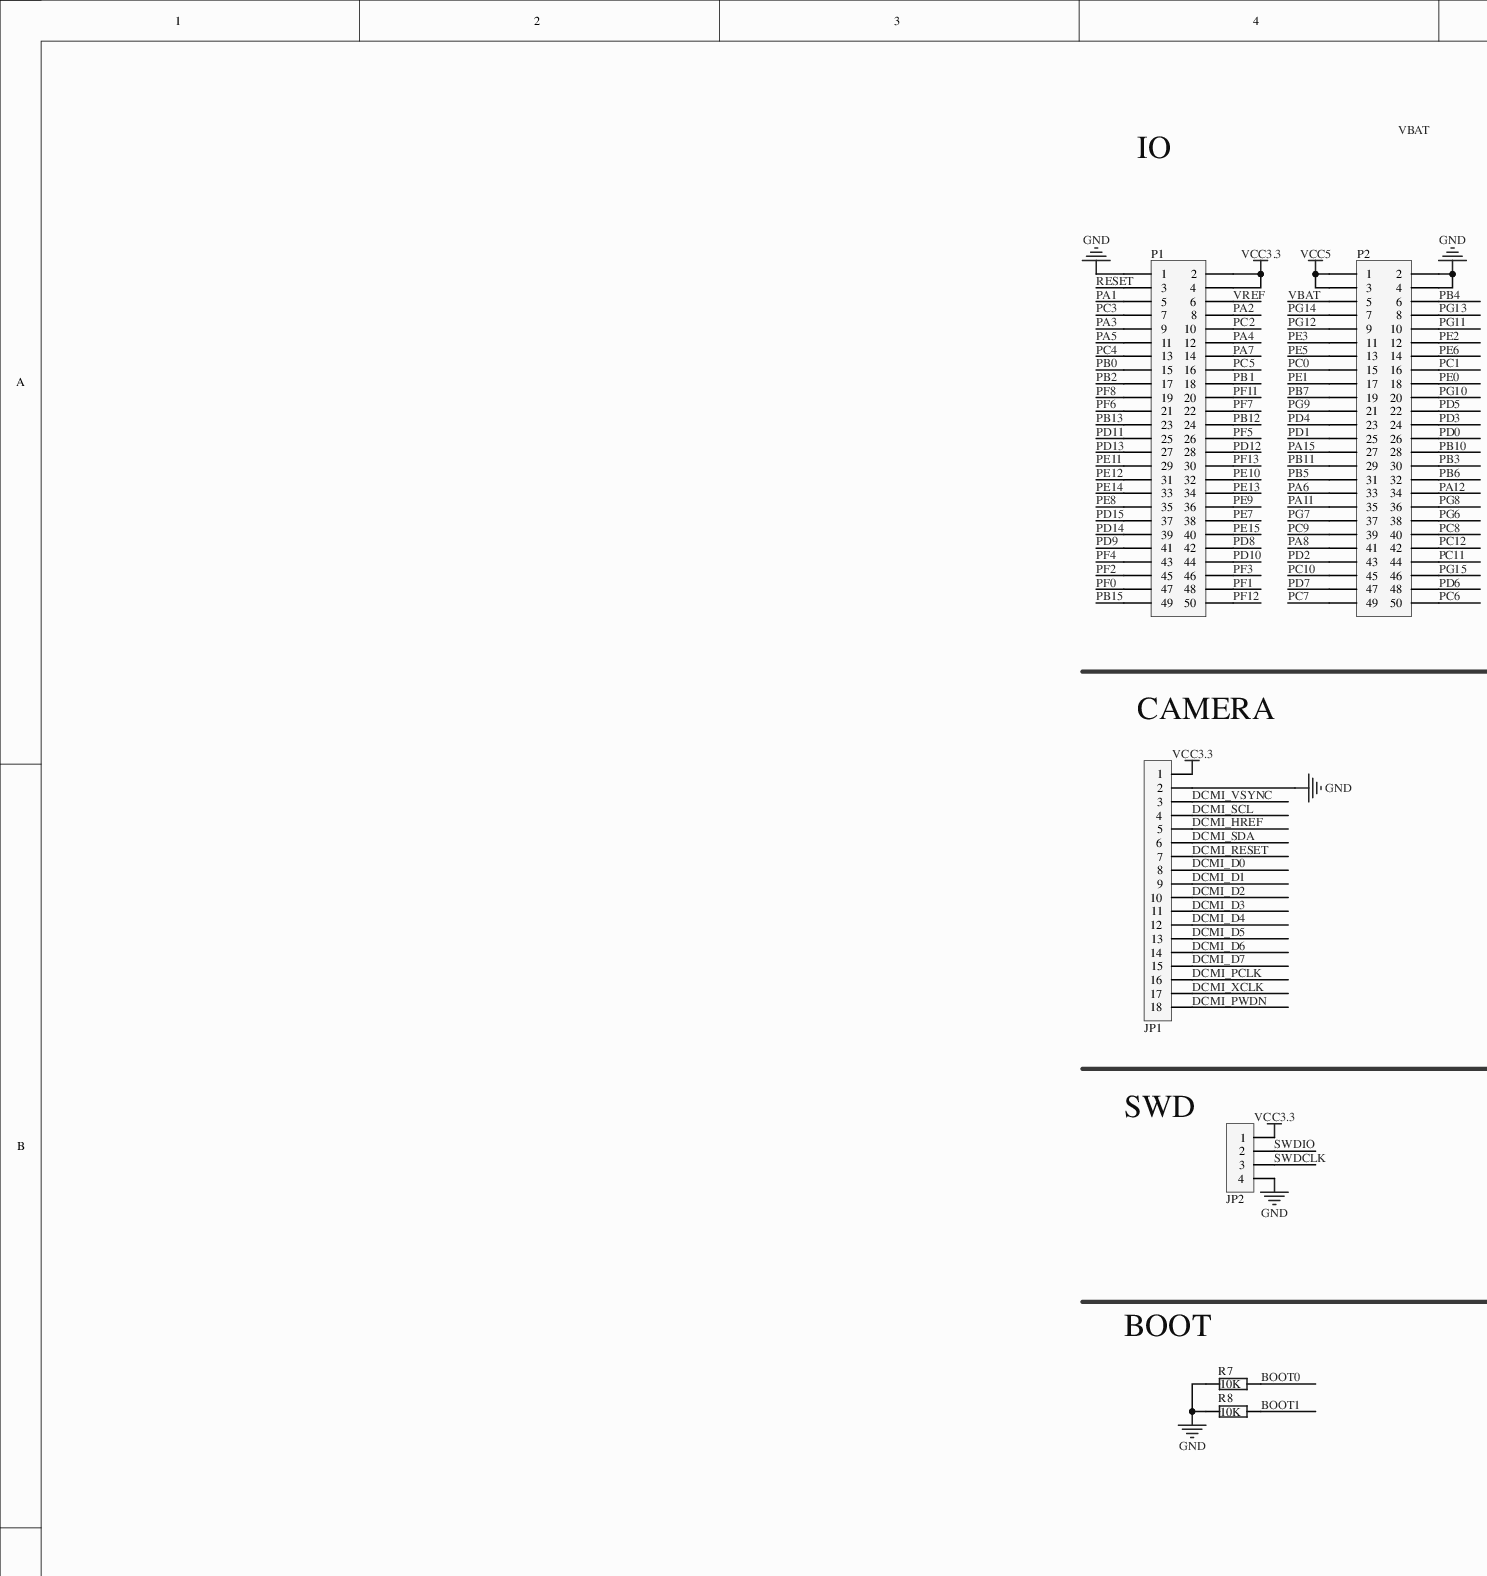
[diagram p0: MISC105440-6.SchDoc, top left]
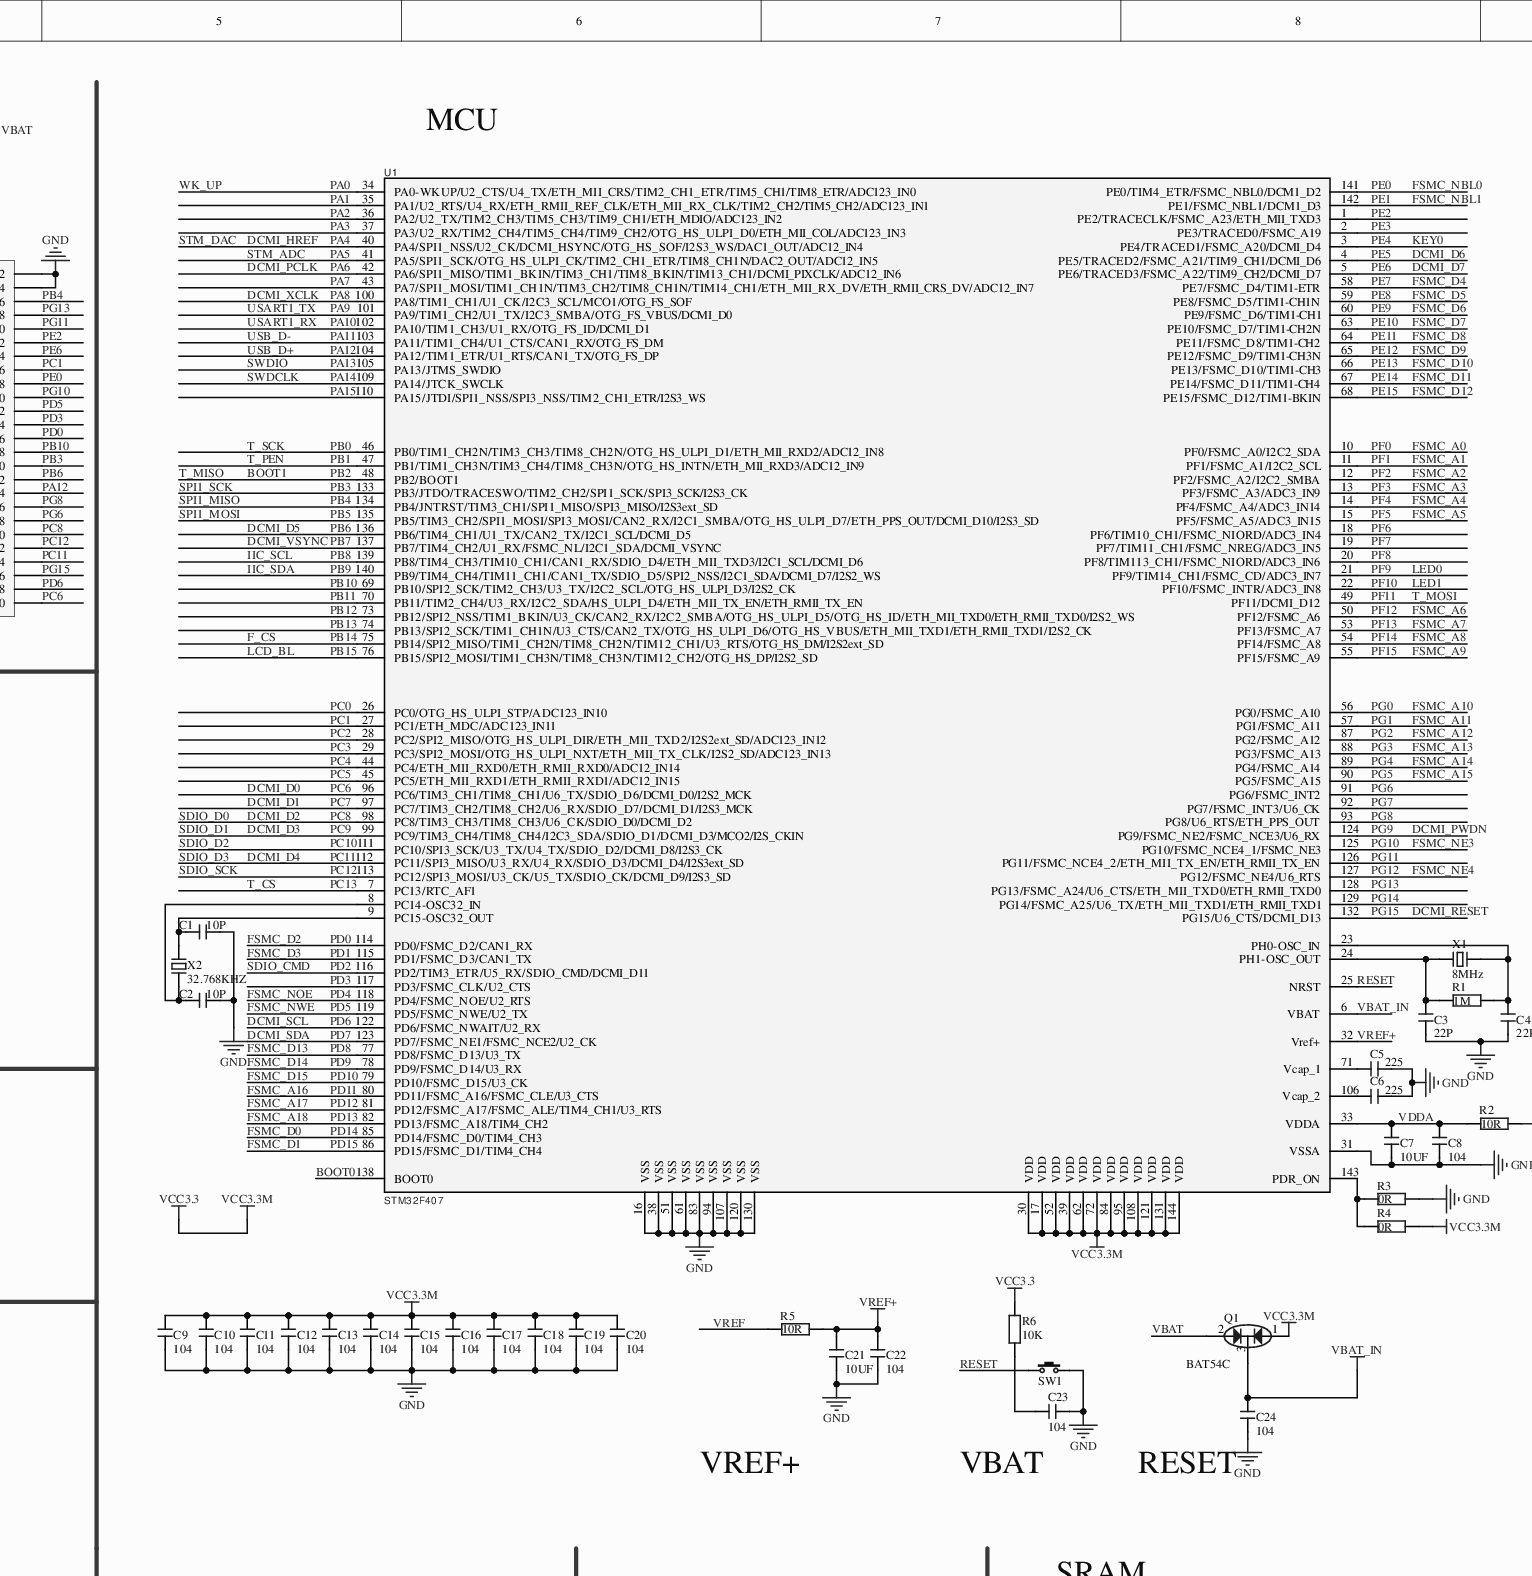
[diagram p1: MISC105440-6.SchDoc, top middle]
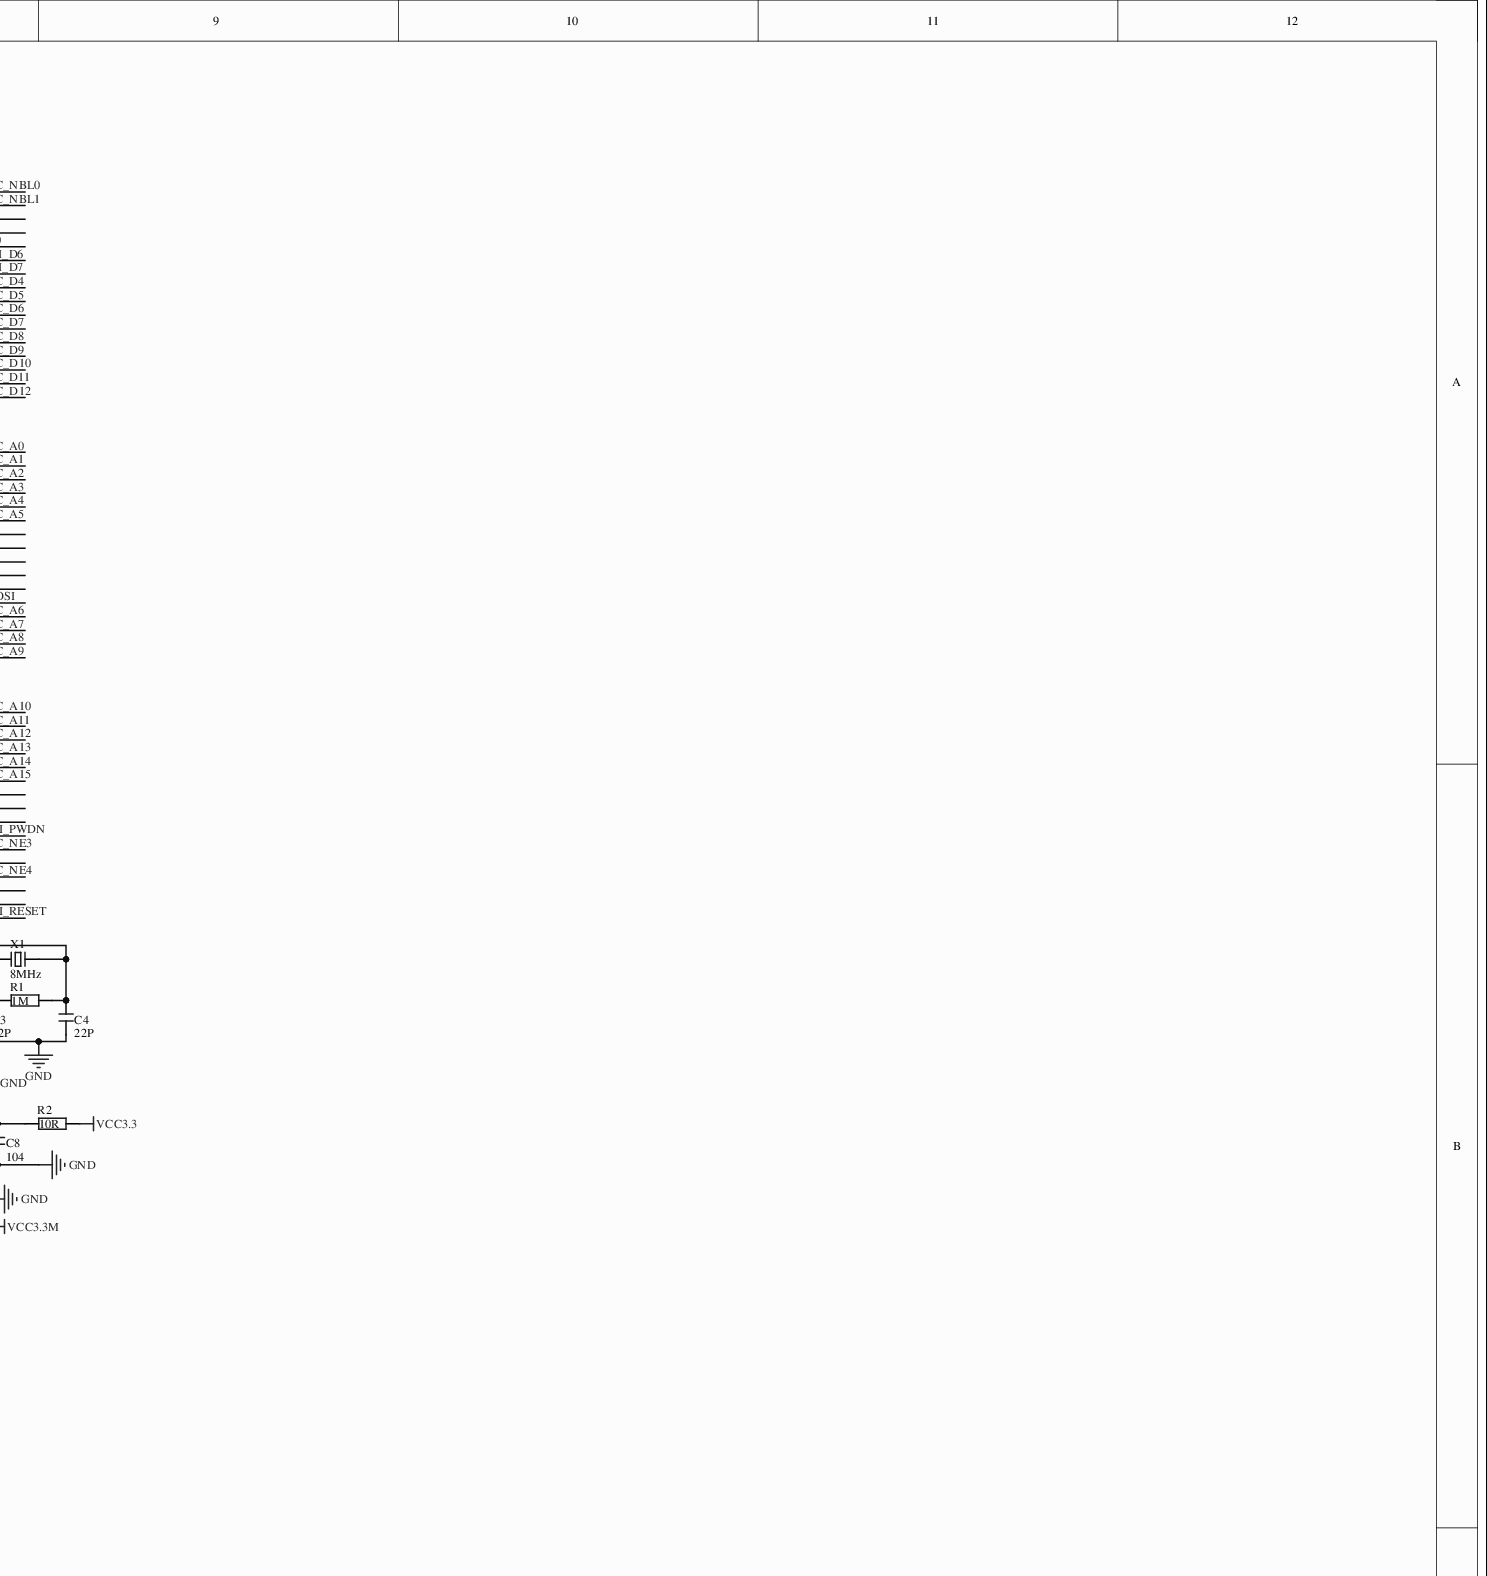
[diagram p2: MISC105440-6.SchDoc, top right]
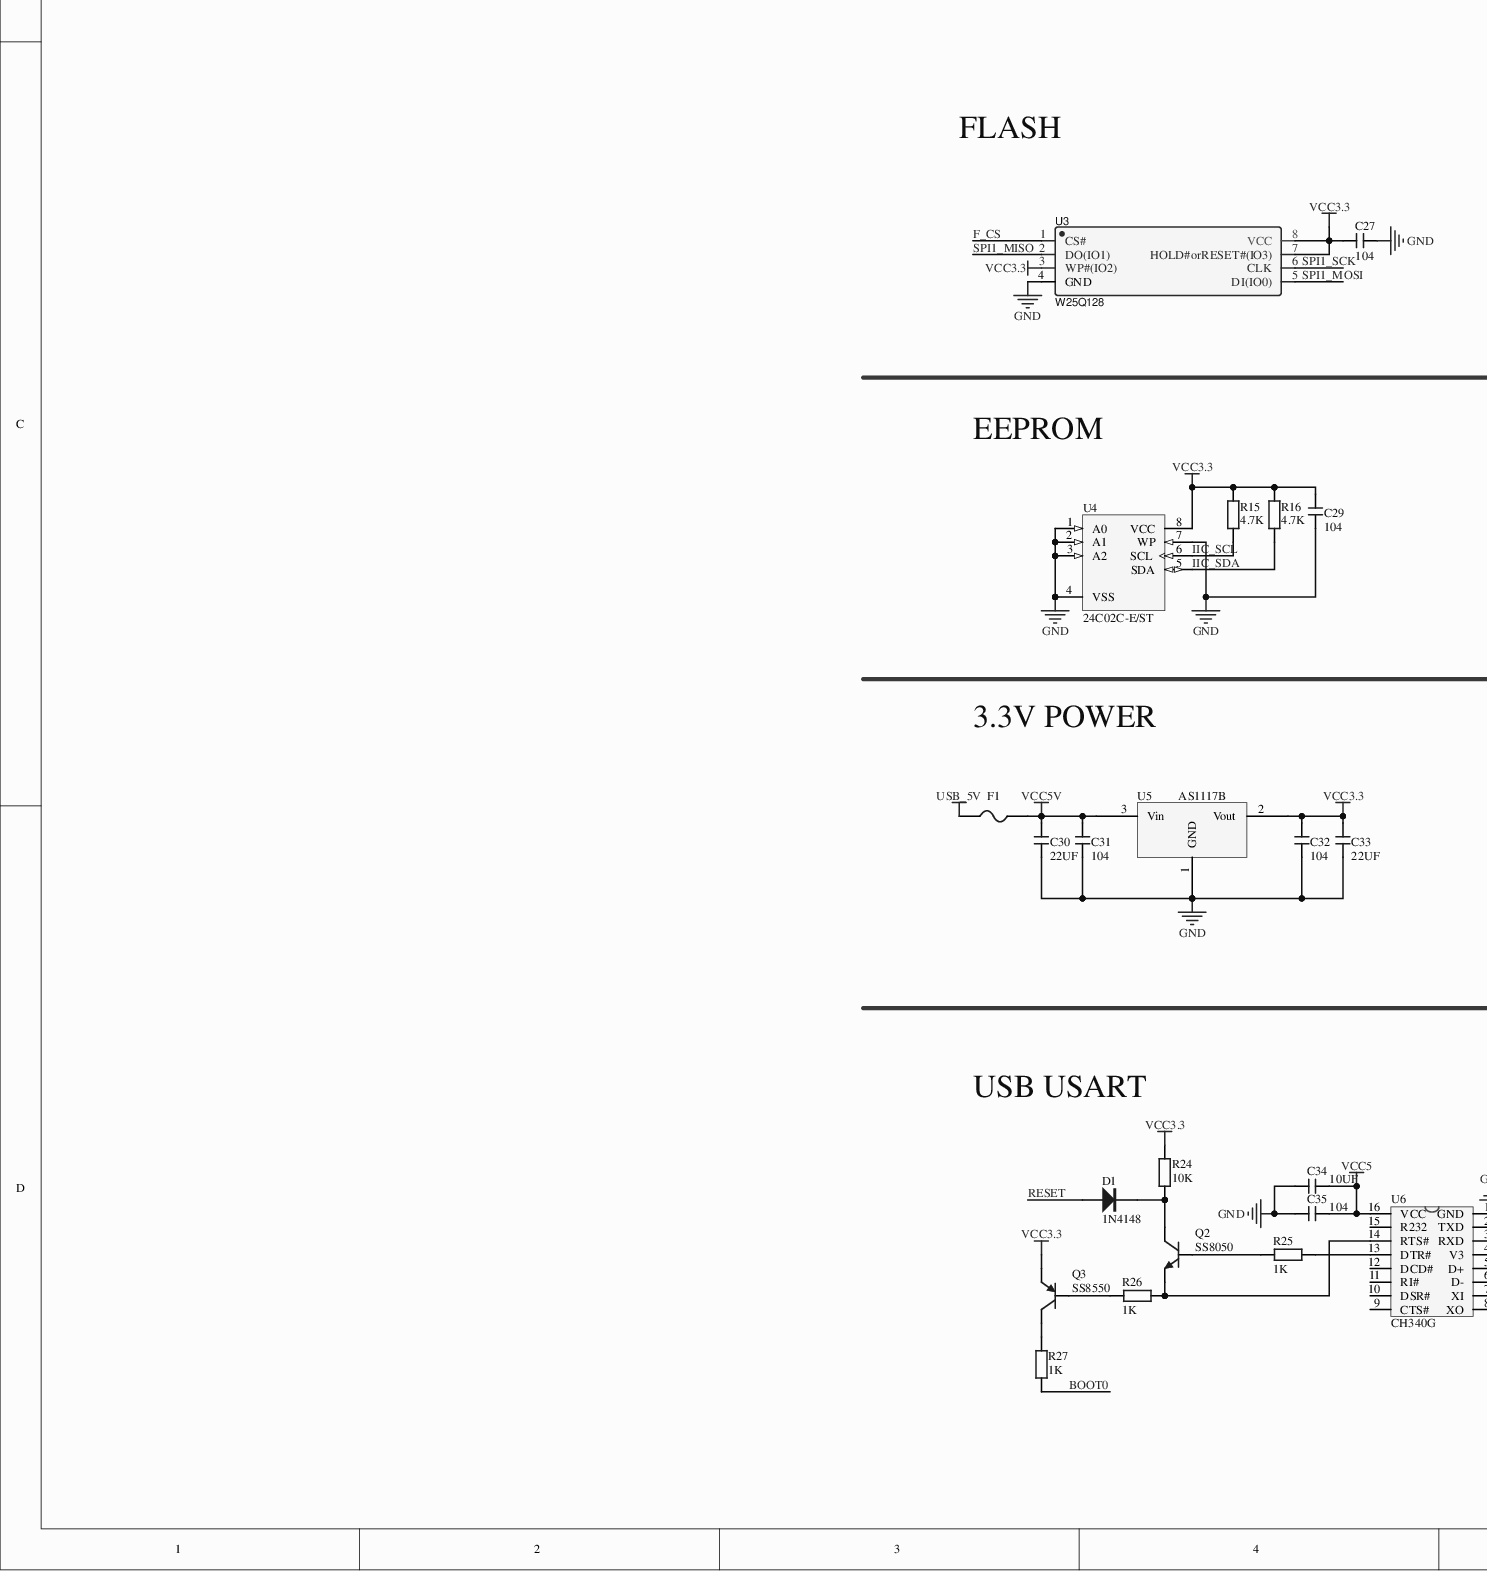
[diagram p3: MISC105440-6.SchDoc, bottom left]
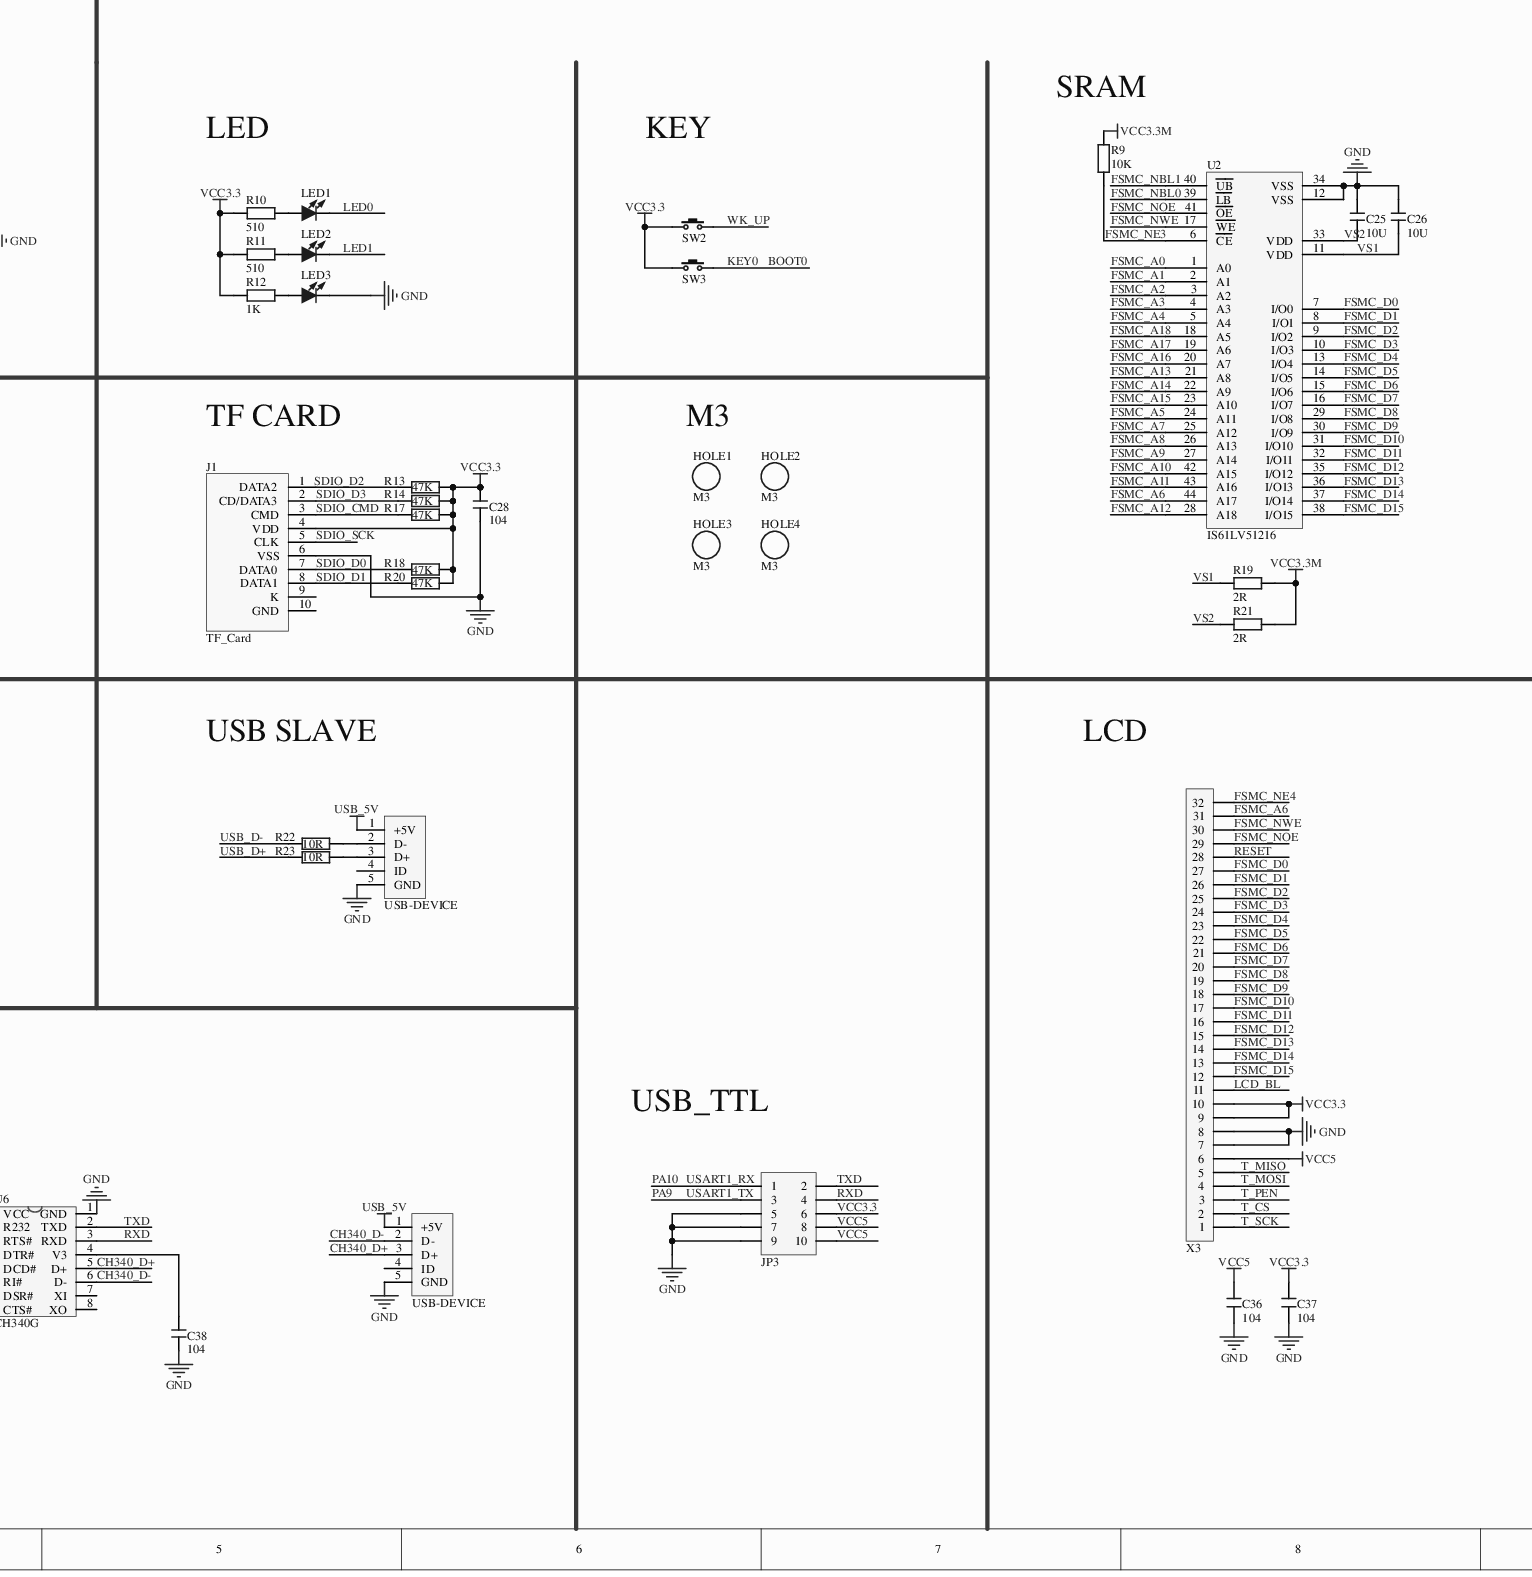
[diagram p4: MISC105440-6.SchDoc, bottom middle]
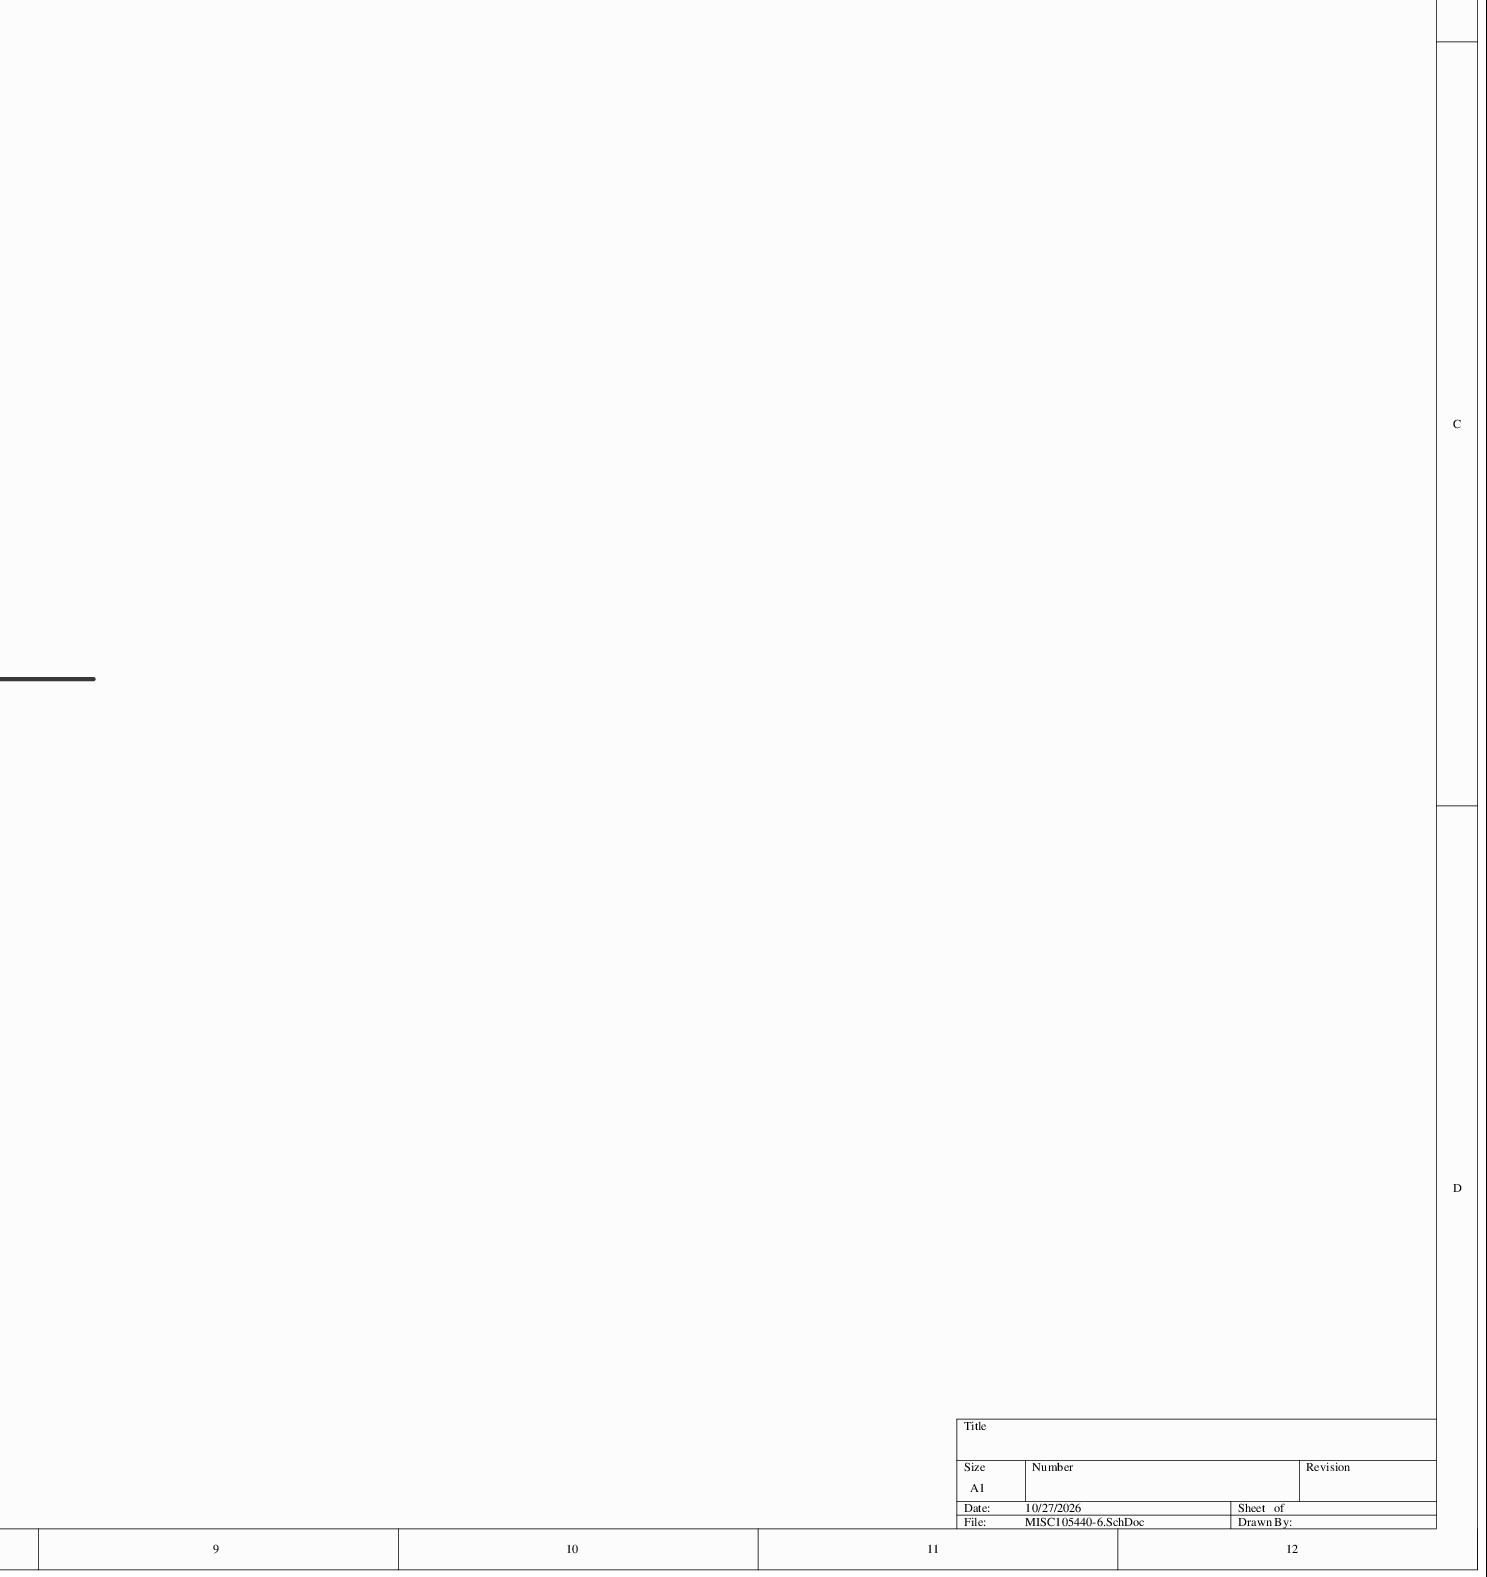
[diagram p5: MISC105440-6.SchDoc, bottom right]
# Altium project MISC105440-4.PrjPcb
1 sheet, 97 parts. Net scope: global (net labels, ports and power ports of the same name join across sheets).
Board file: MISC105440.PcbDoc

## Sheet MISC105440-6.SchDoc
size A1

### Parts
C1  10P  [C 0402]
C2  10P  [C 0402]
C3  22P  [C 0402]
C4  22P  [C 0402]
C5  225  [C 0402]
C6  225  [C 0402]
C7  10UF  [C 0402]
C8  104  [C 0402]
C9  104  [C 0402]
C10  104  [C 0402]
C11  104  [C 0402]
C12  104  [C 0402]
C13  104  [C 0402]
C14  104  [C 0402]
C15  104  [C 0402]
C16  104  [C 0402]
C17  104  [C 0402]
C18  104  [C 0402]
C19  104  [C 0402]
C20  104  [C 0402]
C21  10UF  [C 0402]
C22  104  [C 0402]
C23  104  [C 0402]
C24  104  [C 0402]
C25  10U  [C 0402]
C26  10U  [C 0402]
C27  104  [C 0402]
C28  104  [C 0402]
C29  104  [C 0402]
C30  22UF  [C 0402]
C31  104  [C 0402]
C32  104  [C 0402]
C33  22UF  [C 0402]
C34  10UF  [C 0402]
C35  104  [C 0402]
C36  104  [C 0402]
C37  104  [C 0402]
C38  104  [C 0402]
D1  1N4148  [MINI_MELF (LL34)]
F1  MSMD200-8V 2A  [FU 0805]  (value not drawn)
HOLE1  M3  [M3 5.4MM]
HOLE2  M3  [M3 5.4MM]
HOLE3  M3  [M3 5.4MM]
HOLE4  M3  [M3 5.4MM]
J1  TF_Card  [Micro SD]
JP1  FPC0.5-18P  [FPC0.5 2H-WS-18P]  (value not drawn)
JP2  SWD  [XH2.54-WI-4P]  (value not drawn)
JP3  Header 5X2  [HDR2.54-LI-2x5P]  (value not drawn)
LED1  Red  [LED 0603R]  (value not drawn)
LED2  Red  [LED 0603R]  (value not drawn)
LED3  Red  [LED 0603R]  (value not drawn)
P1  Header 25X2  [HDR2.54-LI-2x25P]  (value not drawn)
P2  Header 25X2  [HDR2.54-LI-2x25P]  (value not drawn)
Q1  BAT54C  [SOT23-3L]
Q2  SS8050  [SOT23-3L]
Q3  SS8550  [SOT23-3L]
R1  1M  [R 0402]
R2  10R  [R 0402]
R3  0R  [R 0402]
R4  0R  [R 0402]
R5  10R  [R 0402]
R6  10K  [R 0402]
R7  10K  [R 0402]
R8  10K  [R 0402]
R9  10K  [R 0402]
R10  510  [R 0402]
R11  510  [R 0402]
R12  1K  [R 0402]
R13  47K  [R 0402]
R14  47K  [R 0402]
R15  4.7K  [R 0402]
R16  4.7K  [R 0402]
R17  47K  [R 0402]
R18  47K  [R 0402]
R19  2R  [R 0402]
R20  47K  [R 0402]
R21  2R  [R 0402]
R22  10R  [R 0402]
R23  10R  [R 0402]
R24  10K  [R 0402]
R25  1K  [R 0402]
R26  1K  [R 0402]
R27  1K  [R 0402]
SW1  3x6x5  [TSW SMD-3*4*2.5]  (value not drawn)
SW2  3x6x5  [TSW SMD-3*4*2.5]  (value not drawn)
SW3  3x6x5  [TSW SMD-3*4*2.5]  (value not drawn)
U1  STM32F407  [LQFP144 20X20_M]
U2  IS61LV51216  [TSOP44_M]
U3  W25Q128  [SOP8W_L]
U4  24C02C-E/ST  [SOP8_L]
U5  AS1117B  [SOT89_L]
U6  CH340G  [SOP16]
USB1  USB-DEVICE  [USB-MICRO_B]
USB2  USB-DEVICE  [USB-MICRO_B]
X1  8MHz  [OSC 5032-2P]
X2  32.768KHZ  [OSC 3215-2P]
X3  FPC0.5-32P  [FPC0.5 2H-WS-32P]  (value not drawn)

### Nets
GND: C1.1 C2.1 C3.1 C4.1 C5.2 C6.2 C7.1 C8.1 C9.1 C10.1 C11.1 C12.1 C13.1 C14.1 C15.1 C16.1 C17.1 C18.1 C19.1 C20.1 C21.2 C22.2 C23.2 C24.1 C25.2 C26.2 C27.2 C28.1 C29.1 C30.1 C31.1 C32.1 C33.1 C34.2 C35.2 C36.1 C37.1 C38.1 J1.6(VSS) JP1.2 JP2.4 JP3.5 JP3.7 JP3.9 LED3.2(K) P1.1 P2.2 P2.4 R3.2 R7.1 R8.1 SW1.2 U1.16(VSS) U1.31(VSSA) U1.38(VSS) U1.51(VSS) U1.61(VSS) U1.83(VSS) U1.94(VSS) U1.107(VSS) U1.120(VSS) U1.130(VSS) U2.12(VSS) U2.34(VSS) U3.4(GND) U4.1(A0) U4.2(A1) U4.3(A2) U4.4(VSS) U4.7(WP) U5.1(GND) U6.1(GND) USB1.5(GND) USB2.5(GND) X3.7 X3.8
USB_5V: F1.1 USB1.1(+5V) USB2.1(+5V)
VBAT_IN: C24.2 Q1.3 U1.6(VBAT)
VCC3.3: C9.2 C10.2 C11.2 C12.2 C13.2 C14.2 C15.2 C16.2 C17.2 C18.2 C19.2 C20.2 C27.1 C28.2 C29.2 C32.2 C33.2 C37.2 J1.4(VDD) JP1.1 JP2.1 JP3.6 P1.2 P1.4 Q1.1 Q3.2(E) R2.2 R4.2 R6.2 R9.2 R10.2 R11.2 R12.2 R13.1 R14.1 R15.2 R16.2 R17.1 R18.1 R19.1 R20.1 R21.1 R24.1 SW2.1 SW3.1 U1.17(VDD) U1.30(VDD) U1.39(VDD) U1.52(VDD) U1.62(VDD) U1.72(VDD) U1.84(VDD) U1.95(VDD) U1.108(VDD) U1.121(VDD) U1.131(VDD) U1.144(VDD) U3.3(WP#(IO2)) U3.7(HOLD#orRESET#(IO3)) U3.8(VCC) U4.8(VCC) U5.2(Vout) X3.9 X3.10  [also labelled VCC3.3M]
VCC5: C34.1 C35.1 C36.2 JP3.8 JP3.10 P2.1 P2.3 U6.16(VCC) X3.6
VCC5V: C30.2 C31.2 F1.2 U5.3(Vin)
VREF+: C21.1 C22.1 R5.2 U1.32(Vref+)
BOOT0: R7.2 R27.2 SW3.2 U1.3(PE4/TRACED1/FSMC_A20/DCMI_D4) U1.138(BOOT0)  [also labelled KEY0, PE4]
BOOT1: P1.17 R8.2 U1.48(PB2/BOOT1) X3.5  [also labelled PB2, T_MISO]
CH340_D+: U6.5(D+) USB2.3(D+)
CH340_D-: U6.6(D-) USB2.2(D-)
DCMI_D0: JP1.8 P2.50 U1.96(PC6/TIM3_CH1/TIM8_CH1/U6_TX/SDIO_D6/DCMI_D0/I2S2_MCK)  [also labelled PC6]
DCMI_D1: JP1.9 P2.49 U1.97(PC7/TIM3_CH2/TIM8_CH2/U6_RX/SDIO_D7/DCMI_D1/I2S3_MCK)  [also labelled PC7]
DCMI_D2: J1.7(DATA0) JP1.10 P2.40 R18.2 U1.98(PC8/TIM3_CH3/TIM8_CH3/U6_CK/SDIO_D0/DCMI_D2)  [also labelled PC8, SDIO_D0]
DCMI_D3: J1.8(DATA1) JP1.11 P2.39 R20.2 U1.99(PC9/TIM3_CH4/TIM8_CH4/I2C3_SDA/SDIO_D1/DCMI_D3/MCO2/I2S_CKIN)  [also labelled PC9, SDIO_D1]
DCMI_D4: J1.2(CD/DATA3) JP1.12 P2.44 R14.2 U1.112(PC11/SPI3_MISO/U3_RX/U4_RX/SDIO_D3/DCMI_D4/I2S3ext_SD)  [also labelled PC11, SDIO_D3]
DCMI_D5: JP1.13 P2.32 U1.136(PB6/TIM4_CH1/U1_TX/CAN2_TX/I2C1_SCL/DCMI_D5)  [also labelled PB6]
DCMI_D6: JP1.14 P2.13 U1.4(PE5/TRACED2/FSMC_A21/TIM9_CH1/DCMI_D6)  [also labelled PE5]
DCMI_D7: JP1.15 P2.14 U1.5(PE6/TRACED3/FSMC_A22/TIM9_CH2/DCMI_D7)  [also labelled PE6]
DCMI_HREF: JP1.5 P1.12 U1.40(PA4/SPI1_NSS/U2_CK/DCMI_HSYNC/OTG_HS_SOF/I2S3_WS/DAC1_OUT/ADC12_IN4)  [also labelled PA4, STM_DAC]
DCMI_PCLK: JP1.16 P2.33 U1.42(PA6/SPI1_MISO/TIM1_BKIN/TIM3_CH1/TIM8_BKIN/TIM13_CH1/DCMI_PIXCLK/ADC12_IN6)  [also labelled PA6]
DCMI_PWDN: JP1.18 P2.21 U1.124(PG9/FSMC_NE2/FSMC_NCE3/U6_RX)  [also labelled PG9]
DCMI_RESET: JP1.7 P2.46 U1.132(PG15/U6_CTS/DCMI_D13)  [also labelled PG15]
DCMI_SCL: JP1.4 P2.48 U1.122(PD6/FSMC_NWAIT/U2_RX)  [also labelled PD6]
DCMI_SDA: JP1.6 P2.47 U1.123(PD7/FSMC_NE1/FSMC_NCE2/U2_CK)  [also labelled PD7]
DCMI_VSYNC: JP1.3 P2.19 U1.137(PB7/TIM4_CH2/U1_RX/FSMC_NL/I2C1_SDA/DCMI_VSYNC)  [also labelled PB7]
DCMI_XCLK: JP1.17 P2.41 U1.100(PA8/TIM1_CH1/U1_CK/I2C3_SCL/MCO1/OTG_FS_SOF)  [also labelled PA8]
F_CS: U1.75(PB14/SPI2_MISO/TIM1_CH2N/TIM8_CH2N/TIM12_CH1/U3_RTS/OTG_HS_DM/I2S2ext_SD) U3.1(CS#)  [also labelled PB14]
FSMC_A0: P1.47 U1.10(PF0/FSMC_A0/I2C2_SDA) U2.1(A0)  [also labelled PF0]
FSMC_A1: P1.48 U1.11(PF1/FSMC_A1/I2C2_SCL) U2.2(A1)  [also labelled PF1]
FSMC_A2: P1.45 U1.12(PF2/FSMC_A2/I2C2_SMBA) U2.3(A2)  [also labelled PF2]
FSMC_A3: P1.46 U1.13(PF3/FSMC_A3/ADC3_IN9) U2.4(A3)  [also labelled PF3]
FSMC_A4: P1.43 U1.14(PF4/FSMC_A4/ADC3_IN14) U2.5(A4)  [also labelled PF4]
FSMC_A5: P1.26 U1.15(PF5/FSMC_A5/ADC3_IN15) U2.24(A11)  [also labelled PF5]
FSMC_A6: P1.50 U1.50(PF12/FSMC_A6) U2.44(A17) X3.31  [also labelled PF12]
FSMC_A7: P1.30 U1.53(PF13/FSMC_A7) U2.25(A12)  [also labelled PF13]
FSMC_A8: U1.54(PF14/FSMC_A8) U2.26(A13)  [also labelled PF14]
FSMC_A9: U1.55(PF15/FSMC_A9) U2.27(A14)  [also labelled PF15]
FSMC_A10: U1.56(PG0/FSMC_A10) U2.42(A15)  [also labelled PG0]
FSMC_A11: U1.57(PG1/FSMC_A11) U2.43(A16)  [also labelled PG1]
FSMC_A12: U1.87(PG2/FSMC_A12) U2.28(A18)  [also labelled PG2]
FSMC_A13: U1.88(PG3/FSMC_A13) U2.21(A8)  [also labelled PG3]
FSMC_A14: U1.89(PG4/FSMC_A14) U2.22(A9)  [also labelled PG4]
FSMC_A15: U1.90(PG5/FSMC_A15) U2.23(A10)  [also labelled PG5]
FSMC_A16: P1.25 U1.80(PD11/FSMC_A16/FSMC_CLE/U3_CTS) U2.20(A7)  [also labelled PD11]
FSMC_A17: P1.28 U1.81(PD12/FSMC_A17/FSMC_ALE/TIM4_CH1/U3_RTS) U2.19(A6)  [also labelled PD12]
FSMC_A18: P1.27 U1.82(PD13/FSMC_A18/TIM4_CH2) U2.18(A5)  [also labelled PD13]
FSMC_D0: P1.39 U1.85(PD14/FSMC_D0/TIM4_CH3) U2.7(I/O0) X3.27  [also labelled PD14]
FSMC_D1: P1.37 U1.86(PD15/FSMC_D1/TIM4_CH4) U2.8(I/O1) X3.26  [also labelled PD15]
FSMC_D2: P2.26 U1.114(PD0/FSMC_D2/CAN1_RX) U2.9(I/O2) X3.25  [also labelled PD0]
FSMC_D3: P2.25 U1.115(PD1/FSMC_D3/CAN1_TX) U2.10(I/O3) X3.24  [also labelled PD1]
FSMC_D4: P1.38 U1.58(PE7/FSMC_D4/TIM1-ETR) U2.13(I/O4) X3.23  [also labelled PE7]
FSMC_D5: P1.35 U1.59(PE8/FSMC_D5/TIM1-CH1N) U2.14(I/O5) X3.22  [also labelled PE8]
FSMC_D6: P1.36 U1.60(PE9/FSMC_D6/TIM1-CH1) U2.15(I/O6) X3.21  [also labelled PE9]
FSMC_D7: P1.32 U1.63(PE10/FSMC_D7/TIM1-CH2N) U2.16(I/O7) X3.20  [also labelled PE10]
FSMC_D8: P1.29 U1.64(PE11/FSMC_D8/TIM1-CH2) U2.29(I/O8) X3.19  [also labelled PE11]
FSMC_D9: P1.31 U1.65(PE12/FSMC_D9/TIM1-CH3N) U2.30(I/O9) X3.18  [also labelled PE12]
FSMC_D10: P1.34 U1.66(PE13/FSMC_D10/TIM1-CH3) U2.31(I/O10) X3.17  [also labelled PE13]
FSMC_D11: P1.33 U1.67(PE14/FSMC_D11/TIM1-CH4) U2.32(I/O11) X3.16  [also labelled PE14]
FSMC_D12: P1.40 U1.68(PE15/FSMC_D12/TIM1-BKIN) U2.35(I/O12) X3.15  [also labelled PE15]
FSMC_D13: P1.42 U1.77(PD8/FSMC_D13/U3_TX) U2.36(I/O13) X3.14  [also labelled PD8]
FSMC_D14: P1.41 U1.78(PD9/FSMC_D14/U3_RX) U2.37(I/O14) X3.13  [also labelled PD9]
FSMC_D15: P1.44 U1.79(PD10/FSMC_D15/U3_CK) U2.38(I/O15) X3.12  [also labelled PD10]
FSMC_NBL0: P2.18 U1.141(PE0/TIM4_ETR/FSMC_NBL0/DCM1_D2) U2.39(~{LB})  [also labelled PE0]
FSMC_NBL1: P2.17 U1.142(PE1/FSMC_NBL1/DCM1_D3) U2.40(~{UB})  [also labelled PE1]
FSMC_NE3: P2.20 R9.1 U1.125(PG10/FSMC_NCE4_1/FSMC_NE3) U2.6(~{CE})  [also labelled PG10]
FSMC_NE4: P2.9 U1.127(PG12/FSMC_NE4/U6_RTS) X3.32  [also labelled PG12]
FSMC_NOE: P2.23 U1.118(PD4/FSMC_NOE/U2_RTS) U2.41(~{OE}) X3.29  [also labelled PD4]
FSMC_NWE: P2.22 U1.119(PD5/FSMC_NWE/U2_TX) U2.17(~{WE}) X3.30  [also labelled PD5]
IIC_SCL: R15.1 U1.139(PB8/TIM4_CH3/TIM10_CH1/CAN1_RX/SDIO_D4/ETH_MII_TXD3/I2C1_SCL/DCMI_D6) U4.6(SCL)  [also labelled PB8]
IIC_SDA: R16.1 U1.140(PB9/TIM4_CH4/TIM11_CH1/CAN1_TX/SDIO_D5/SPI2_NSS/I2C1_SDA/DCMI_D7/I2S2_WS) U4.5(SDA)  [also labelled PB9]
LCD_BL: P1.49 U1.76(PB15/SPI2_MOSI/TIM1_CH3N/TIM8_CH3N/TIM12_CH2/OTG_HS_DP/I2S2_SD) X3.11  [also labelled PB15]
LED0: LED1.2(K) U1.21(PF9/TIM14_CH1/FSMC_CD/ADC3_IN7)  [also labelled PF9]
LED1: LED2.2(K) U1.22(PF10/FSMC_INTR/ADC3_IN8)  [also labelled PF10]
PA0: SW2.2 U1.34(PA0-WKUP/U2_CTS/U4_TX/ETH_MII_CRS/TIM2_CH1_ETR/TIM5_CH1/TIM8_ETR/ADC123_IN0)  [also labelled WK_UP]
PA1: P1.5 U1.35(PA1/U2_RTS/U4_RX/ETH_RMII_REF_CLK/ETH_MII_RX_CLK/TIM2_CH2/TIM5_CH2/ADC123_IN1)
PA2: P1.8 U1.36(PA2/U2_TX/TIM2_CH3/TIM5_CH3/TIM9_CH1/ETH_MDIO/ADC123_IN2)
PA3: P1.9 U1.37(PA3/U2_RX/TIM2_CH4/TIM5_CH4/TIM9_CH2/OTG_HS_ULPI_D0/ETH_MII_COL/ADC123_IN3)
PA5: P1.11 U1.41(PA5/SPI1_SCK/OTG_HS_ULPI_CK/TIM2_CH1_ETR/TIM8_CH1N/DAC2_OUT/ADC12_IN5)  [also labelled STM_ADC]
PA7: P1.14 U1.43(PA7/SPI1_MOSI/TIM1_CH1N/TIM3_CH2/TIM8_CH1N/TIM14_CH1/ETH_MII_RX_DV/ETH_RMII_CRS_DV/ADC12_IN7)
PA9: JP3.3 U1.101(PA9/TIM1_CH2/U1_TX/I2C3_SMBA/OTG_FS_VBUS/DCMI_D0)  [also labelled USART1_TX]
PA10: JP3.1 U1.102(PA10/TIM1_CH3/U1_RX/OTG_FS_ID/DCMI_D1)  [also labelled USART1_RX]
PA11: P2.35 R22.2 U1.103(PA11/TIM1_CH4/U1_CTS/CAN1_RX/OTG_FS_DM)  [also labelled USB_D-]
PA12: P2.34 R23.2 U1.104(PA12/TIM1_ETR/U1_RTS/CAN1_TX/OTG_FS_DP)  [also labelled USB_D+]
PA13: JP2.2 U1.105(PA13/JTMS_SWDIO)  [also labelled SWDIO]
PA14: JP2.3 U1.109(PA14/JTCK_SWCLK)  [also labelled SWDCLK]
PA15: P2.27 U1.110(PA15/JTDI/SPI1_NSS/SPI3_NSS/TIM2_CH1_ETR/I2S3_WS)
PB0: P1.15 U1.46(PB0/TIM1_CH2N/TIM3_CH3/TIM8_CH2N/OTG_HS_ULPI_D1/ETH_MII_RXD2/ADC12_IN8) X3.1  [also labelled T_SCK]
PB1: P1.18 U1.47(PB1/TIM1_CH3N/TIM3_CH4/TIM8_CH3N/OTG_HS_INTN/ETH_MII_RXD3/ADC12_IN9) X3.3  [also labelled T_PEN]
PB3: P2.30 U1.133(PB3/JTDO/TRACESWO/TIM2_CH2/SPI1_SCK/SPI3_SCK/I2S3_CK) U3.6(CLK)  [also labelled SPI1_SCK]
PB4: P2.6 U1.134(PB4/JNTRST/TIM3_CH1/SPI1_MISO/SPI3_MISO/I2S3ext_SD) U3.2(DO(IO1))  [also labelled SPI1_MISO]
PB5: P2.31 U1.135(PB5/TIM3_CH2/SPI1_MOSI/SPI3_MOSI/CAN2_RX/I2C1_SMBA/OTG_HS_ULPI_D7/ETH_PPS_OUT/DCMI_D10/I2S3_SD) U3.5(DI(IO0))  [also labelled SPI1_MOSI]
PB10: P2.28 U1.69(PB10/SPI2_SCK/TIM2_CH3/U3_TX/I2C2_SCL/OTG_HS_ULPI_D3/I2S2_CK)
PB11: P2.29 U1.70(PB11/TIM2_CH4/U3_RX/I2C2_SDA/HS_ULPI_D4/ETH_MII_TX_EN/ETH_RMII_TX_EN)
PB12: P1.24 U1.73(PB12/SPI2_NSS/TIM1_BKIN/U3_CK/CAN2_RX/I2C2_SMBA/OTG_HS_ULPI_D5/OTG_HS_ID/ETH_MII_TXD0/ETH_RMII_TXD0/I2S2_WS)
PB13: P1.23 U1.74(PB13/SPI2_SCK/TIM1_CH1N/U3_CTS/CAN2_TX/OTG_HS_ULPI_D6/OTG_HS_VBUS/ETH_MII_TXD1/ETH_RMII_TXD1/I2S2_CK)
PC0: P2.15 U1.26(PC0/OTG_HS_ULPI_STP/ADC123_IN10)
PC1: P2.16 U1.27(PC1/ETH_MDC/ADC123_IN11)
PC2: P1.10 U1.28(PC2/SPI2_MISO/OTG_HS_ULPI_DIR/ETH_MII_TXD2/I2S2ext_SD/ADC123_IN12)
PC3: P1.7 U1.29(PC3/SPI2_MOSI/OTG_HS_ULPI_NXT/ETH_MII_TX_CLK/I2S2_SD/ADC123_IN13)
PC4: P1.13 U1.44(PC4/ETH_MII_RXD0/ETH_RMII_RXD0/ADC12_IN14)
PC5: P1.16 U1.45(PC5/ETH_MII_RXD1/ETH_RMII_RXD1/ADC12_IN15)
PC10: P2.45 U1.111(PC10/SPI3_SCK/U3_TX/U4_TX/SDIO_D2/DCMI_D8/I2S3_CK)  [also labelled SDIO_D2]
PC12: J1.5(CLK) P2.42 U1.113(PC12/SPI3_MOSI/U3_CK/U5_TX/SDIO_CK/DCMI_D9/I2S3_SD)  [also labelled SDIO_SCK]
PC13: U1.7(PC13/RTC_AF1) X3.2  [also labelled T_CS]
PD2: J1.3(CMD) P2.43 R17.2 U1.116(PD2/TIM3_ETR/U5_RX/SDIO_CMD/DCMI_D11)  [also labelled SDIO_CMD]
PD3: P2.24 U1.117(PD3/FSMC_CLK/U2_CTS)
PE2: P2.12 U1.1(PE2/TRACECLK/FSMC_A23/ETH_MII_TXD3)
PE3: P2.11 U1.2(PE3/TRACED0/FSMC_A19)
PF6: P1.21 U1.18(PF6/TIM10_CH1/FSMC_NIORD/ADC3_IN4)
PF7: P1.22 U1.19(PF7/TIM11_CH1/FSMC_NREG/ADC3_IN5)
PF8: P1.19 U1.20(PF8/TIM113_CH1/FSMC_NIORD/ADC3_IN6)
PF11: P1.20 U1.49(PF11/DCMI_D12) X3.4  [also labelled T_MOSI]
PG6: P2.38 U1.91(PG6/FSMC_INT2)
PG7: P2.37 U1.92(PG7/FSMC_INT3/U6_CK)
PG8: P2.36 U1.93(PG8/U6_RTS/ETH_PPS_OUT)
PG11: P2.10 U1.126(PG11/FSMC_NCE4_2/ETH_MII_TX_EN/ETH_RMII_TX_EN)
PG13: P2.8 U1.128(PG13/FSMC_A24/U6_CTS/ETH_MII_TXD0/ETH_RMII_TXD0)
PG14: P2.7 U1.129(PG14/FSMC_A25/U6_TX/ETH_MII_TXD1/ETH_RMII_TXD1)
RESET: D1.1(A) P1.3 SW1.1 U1.25(NRST) X3.28
RXD: JP3.4 U6.3(RXD)
TXD: JP3.2 U6.2(TXD)
VBAT: P2.5 Q1.2
VDDA: C7.2 C8.2 R2.1 U1.33(VDDA)
VREF: P1.6 R5.1
VS1: C26.1 R19.2 U2.11(VDD)
VS2: C25.1 R21.2 U2.33(VDD)
NetC1_2: C1.2 U1.9(PC15-OSC32_OUT) X2.2
NetC2_2: C2.2 U1.8(PC14-OSC32_IN) X2.1
NetC3_2: C3.2 R1.1 U1.24(PH1-OSC_OUT) X1.1
NetC4_2: C4.2 R1.2 U1.23(PH0-OSC_IN) X1.2
NetC5_1: C5.1 U1.71(Vcap_1)
NetC6_1: C6.1 U1.106(Vcap_2)
NetC23_1: C23.1 R6.1
NetC38_2: C38.2 U6.4(V3)
NetD1_2: D1.2(K) Q2.3(C) R24.2
NetJ1_1: J1.1(DATA2) R13.2
NetLED1_1: LED1.1(A) R10.1
NetLED2_1: LED2.1(A) R11.1
NetLED3_1: LED3.1(A) R12.1
NetQ2_1: Q2.1(B) R25.2
NetQ2_2: Q2.2(E) R26.1 U6.14(RTS#)
NetQ3_1: Q3.1(B) R26.2
NetQ3_3: Q3.3(C) R27.1
NetR3_1: R3.1 R4.1 U1.143(PDR_ON)
NetR22_1: R22.1 USB1.2(D-)
NetR23_1: R23.1 USB1.3(D+)
NetR25_1: R25.1 U6.13(DTR#)

Not connected (* = marked no-connect by the designer): J1 9(K)* 10(GND)*; U6 7(XI) 8(XO) 9(CTS#) 10(DSR#) 11(RI#) 12(DCD#) 15(R232); USB1 4(ID); USB2 4(ID)

### Notes on the sheet
- MCU
- IO
- (near JP1) CAMERA
- SWD
- BOOT
- VREF+
- (near C23) VBAT
- (near C24) RESET
- FLASH
- LED
- KEY
- (near R9) SRAM
- TF CARD
- (near HOLE1) M3
- EEPROM
- 3.3V POWER
- USB SLAVE
- LCD
- USB USART
- USB_TTL
- Labels drawn without touching a wire or pin: SDIO_D2, VBAT

### Library data of the parts
C1-C35 C38 = C: SMD capacitor; BOM名称: Non-polar SMD capacitor
C36 C37 = C: Non-polar SMD capacitor; 版权归属: COMPANY_B; 材质: X7R; BOM名称: Non-polar SMD capacitor
D1 = 1N4148: Switching diode; BOM名称: High-speed switching diode
F1 = FU: SMD fuse; BOM名称: SMD fuse
HOLE1-HOLE4 = M3: Copper pillar hole; 版权归属: COMPANY_B; BOM名称: Copper pillar hole
J1 = TF_Card: TF card socket; 版权归属: COMPANY_B; BOM名称: TF card socket
JP1 = FPC-18P: FPC connector; 版权归属: COMPANY_B; BOM名称: FPC connector
JP2 = Header 4: 4P connector; 版权归属: COMPANY_B; BOM名称: 4P connector
JP3 = Header 5X2: 5*2P connector; 版权归属: COMPANY_B; BOM名称: 5*2P connector
LED1-LED3 = LED-SMD: SMD LED; BOM名称: SMD LED
P1 P2 = Header 25X2: Header, 25-Pin, Dual row; LatestRevisionDate: 17-Jul-2002; LatestRevisionNote: Re-released for DXP Platform.; Publisher: Altium Limited
Q1 = BAT54C: SMD Schottky diode; 版权归属: COMPANY_B; 属性: 30V/0.2A; BOM名称: Schottky diode
Q2 = 8050-SMD: RF amplifier, NPN type; 版权归属: COMPANY_B; 属性: 40V 1.5A 1W 100MHZ; BOM名称: RF amplifier, NPN type
Q3 = 8550-SMD: RF amplifier, PNP type; 版权归属: COMPANY_B; 属性: 40V 1.5A 1W 100MHZ; BOM名称: RF amplifier, PNP type
R1-R27 = R: SMD resistor; BOM名称: SMD resistor
SW1-SW3 = TSW 3x6: 3x6 tactile switch; BOM名称: 3x6 tactile switch
U2 = IS61LV51216: Static RAM
U4 = 24C02C-E/ST: 2Kbit, 400kHz, 5V, I2C Serial EEPROM, 8-Pin TSSOP, Extended Temperature; Published: 29-Jan-2009; DatasheetVersion: revJ, Aug-2008; PackageVersion: revBB, Aug-2009; PackageReference: TSSOP-ST8; PackageDescription: 8-Lead Plastic Thin Shrink Small Outline (ST) - 4.4mm Body [TSSOP]; Supplier 1: Digi-Key; Supplier Part Number 1: 24C02C-E/ST-ND; Code_JEDEC: MO-153; ComponentLink1Description: Datasheet; ComponentLink1URL: http://ww1.microchip.com/downloads/en/DeviceDoc/21202J.pdf; ComponentLink2Description: Packaging Specification; ComponentLink2URL: http://www.microchip.com/stellent/groups/techpub_sg/documents/packagingspec/en012702.pdf; ComponentLink3Description: Microchip.com Home; Publisher: Altium Limited
U5 = AMS1117: Three-terminal voltage regulator
U6 = CH340G: USB2UART
USB1 USB2 = USB-5P: Micro USB receptacle; 版权归属: COMPANY_B; BOM名称: Micro USB receptacle
X1 X2 = XTAL-2P: 2-pin passive crystal oscillator; BOM名称: 2-pin passive crystal oscillator
X3 = FPC-32P: FPC connector; 版权归属: COMPANY_B; BOM名称: FPC connector